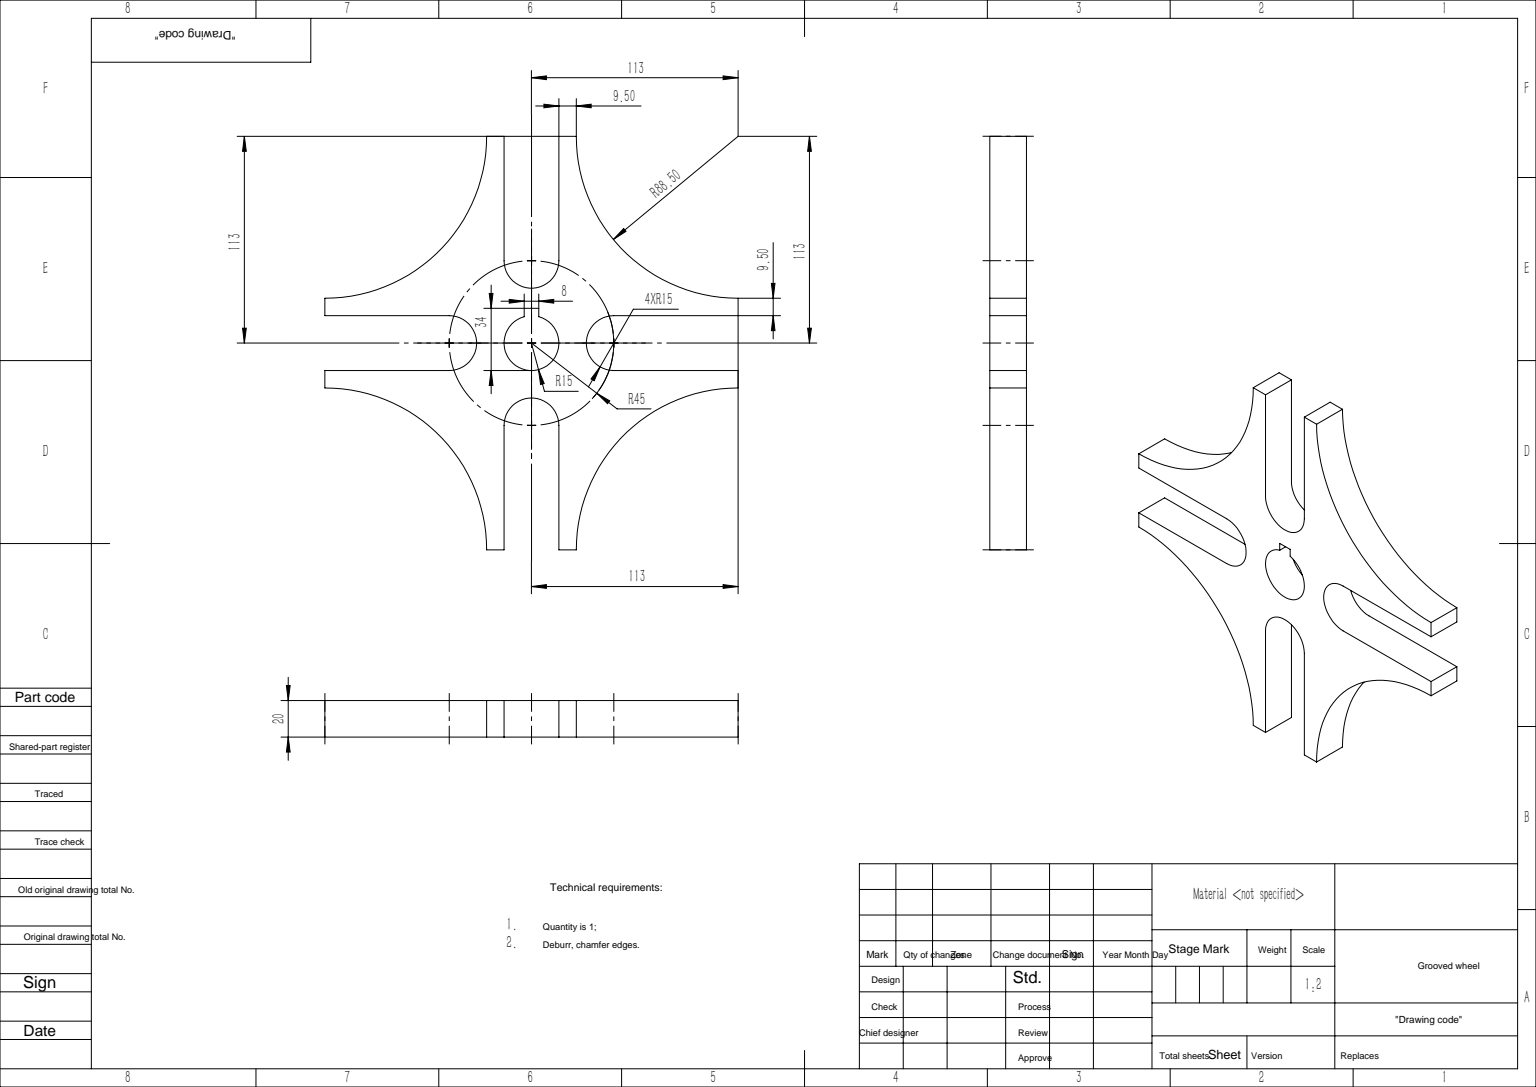
from build123d import *

# Parameters (mm, degrees)
EXTRUDE_1_DEPTH     = 20
CUT_EXTRUDE_1_DEPTH = 162.052786378


with BuildPart() as part:
    # 草图1 → 凸台-拉伸1 (new body)
    with BuildSketch(Plane.XY):
        with BuildLine():
            Line((45, 15), (113, 15))
            Line((113, 15), (113, 24.5))
            ThreePointArc((113, 24.5), (50.421049865, 50.421049865), (24.5, 113))
            Line((24.5, 113), (15, 113))
            Line((15, 113), (15, 45))
            ThreePointArc((15, 45), (10.606601718, 34.393398282), (0, 30))
            ThreePointArc((0, 30), (-10.606601718, 34.393398282), (-15, 45))
            Line((-15, 45), (-15, 113))
            Line((-15, 113), (-24.5, 113))
            ThreePointArc((-24.5, 113), (-50.421049865, 50.421049865), (-113, 24.5))
            Line((-113, 24.5), (-113, 15))
            Line((-113, 15), (-45, 15))
            ThreePointArc((-45, 15), (-34.393398282, 10.606601718), (-30, 0))
            ThreePointArc((-30, 0), (-34.393398282, -10.606601718), (-45, -15))
            Line((-45, -15), (-113, -15))
            Line((-113, -15), (-113, -24.5))
            ThreePointArc((-113, -24.5), (-50.421049865, -50.421049865), (-24.5, -113))
            Line((-24.5, -113), (-15, -113))
            Line((-15, -113), (-15, -45))
            ThreePointArc((-15, -45), (-10.606601718, -34.393398282), (0, -30))
            ThreePointArc((0, -30), (10.606601718, -34.393398282), (15, -45))
            Line((15, -45), (15, -113))
            Line((15, -113), (24.5, -113))
            ThreePointArc((24.5, -113), (50.421049865, -50.421049865), (113, -24.5))
            Line((113, -24.5), (113, -15))
            Line((113, -15), (45, -15))
            ThreePointArc((45, -15), (34.393398282, -10.606601718), (30, 0))
            ThreePointArc((30, 0), (34.393398282, 10.606601718), (45, 15))
        make_face()
    extrude(amount=EXTRUDE_1_DEPTH)

    # 草图2 → 切除-拉伸1 (cut, through all)
    with BuildSketch(Plane.XY.offset(20)):
        with BuildLine():
            Line((-4, 19), (4, 19))
            Line((4, 19), (4, 14.456832295))
            ThreePointArc((4, 14.456832295), (0, -15), (-4, 14.456832295))
            Line((-4, 14.456832295), (-4, 19))
        make_face()
    extrude(amount=-CUT_EXTRUDE_1_DEPTH, mode=Mode.SUBTRACT)


solid = part.part
